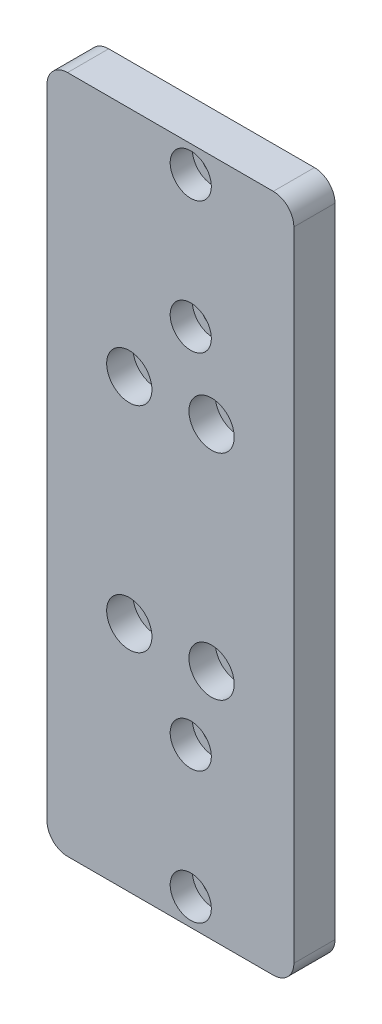
SolidWorks part; units mm, degrees
ref_plane "Front Plane" through (0, 0, 0) normal (0, 0, 1) x (1, 0, 0)
ref_plane "Top Plane" through (0, 0, 0) normal (0, 1, 0) x (1, 0, 0)
ref_plane "Right Plane" through (0, 0, 0) normal (1, 0, 0) x (0, 0, -1)
sketch "Sketch1" plane through (0, 0, 0) normal (0, 0, 1) x (1, 0, 0)
  line L1 (-30, -82.5) -> (30, -82.5)
  line L2 (-30, -82.5) -> (-30, 82.5)
  line L3 (-30, 82.5) -> (30, 82.5)
  line L4 (30, -82.5) -> (30, 82.5)
  line L5 (-30, -82.5) -> (30, 82.5) construction
  line L6 (-30, 82.5) -> (30, -82.5) construction
  point P0 (0, 0)
  dimension "D1" = 60
  dimension "D2" = 165
extrude "Boss-Extrude1" add sketch "Sketch1" along normal blind 10
hole_wizard "CBORE for M6 Hex Socket Head Cap Screw1" positions "Sketch2" profile "Sketch3" counterbore size "M6" standard "ISO" end condition through all
sketch "Sketch2" plane through (0, 0, 10) normal (0, 0, 1) x (1, 0, 0)
  point P0 (-10, 26)
  point P3 (10, 26)
  point P6 (10, -26)
  point P9 (-10, -26)
sketch "Sketch3" plane through (-10, 26, 10) normal (1, 0, 0) x (0, -1, 0)
  line L0 (0, 0) -> (0, 10)
  line L1 (0, 10) -> (3.3, 10)
  line L3 (3.3, 10) -> (3.3, 6.4)
  line L4 (3.3, 6.4) -> (5.5, 6.4)
  line L5 (5.5, 6.4) -> (5.5, 0)
  line L7 (5.5, 0) -> (0, 0)
  line L11 (0, -6.35) -> (0, 107.95) construction
  dimension "通孔孔直径" = 6.6
  dimension "通孔孔深度" = 10
  dimension "柱形沉头孔直径" = 11
  dimension "柱形沉头孔深度" = 6.4
hole_wizard "CBORE for M5 Hex Socket Head Cap Screw2" positions "Sketch6" profile "Sketch7" counterbore size "M5" standard "ISO" end condition through all
sketch "Sketch6" plane through (0, 0, 10) normal (0, 0, 1) x (1, 0, 0)
  point P0 (4.943, 76)
  point P3 (4.943, 44)
  point P6 (4.943, -44)
  point P9 (4.943, -76)
sketch "Sketch7" plane through (4.943, 76, 10) normal (1, 0, 0) x (0, -1, 0)
  line L0 (0, 0) -> (0, 10)
  line L1 (0, 10) -> (2.75, 10)
  line L3 (2.75, 10) -> (2.75, 5.4)
  line L4 (2.75, 5.4) -> (5, 5.4)
  line L5 (5, 5.4) -> (5, 0)
  line L7 (5, 0) -> (0, 0)
  line L11 (0, -6.35) -> (0, 107.95) construction
  dimension "通孔孔直径" = 5.5
  dimension "通孔孔深度" = 10
  dimension "柱形沉头孔直径" = 10
  dimension "柱形沉头孔深度" = 5.4
fillet "Fillet1" radius 5 4 edges at (-30, 82.5, 5) (30, 82.5, 5) (30, -82.5, 5) (-30, -82.5, 5)
